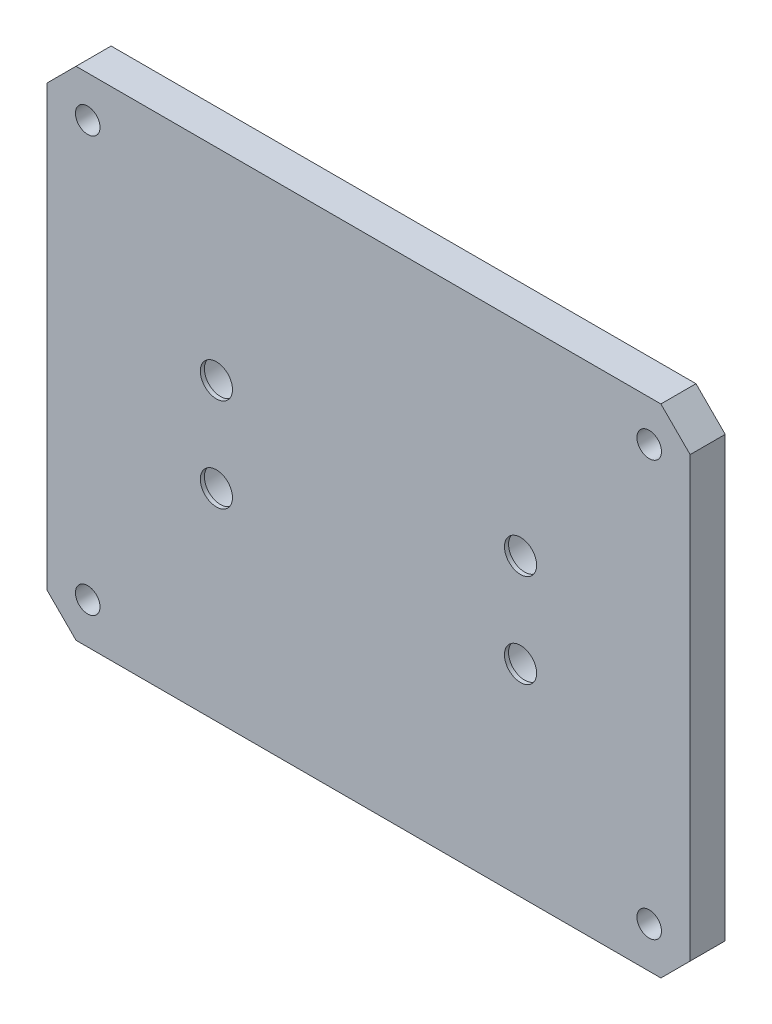
SolidWorks part; units mm, degrees
material "6061-T6 (SS)"
ref_plane "前视基准面" through (0, 0, 0) normal (0, 0, 1) x (1, 0, 0)
ref_plane "上视基准面" through (0, 0, 0) normal (0, 1, 0) x (1, 0, 0)
ref_plane "右视基准面" through (0, 0, 0) normal (1, 0, 0) x (0, 0, -1)
sketch "草图1" plane through (0, 0, 0) normal (0, 0, 1) x (1, 0, 0)
  line L1 (-76.0336, 31.3849) -> (33.9664, 31.3849)
  line L2 (-76.0336, 31.3849) -> (-76.0336, -53.6151)
  line L3 (-76.0336, -53.6151) -> (33.9664, -53.6151)
  line L4 (33.9664, 31.3849) -> (33.9664, -53.6151)
extrude "凸台-拉伸1" add sketch "草图1" along normal blind 6
chamfer "倒角1" distance 5 angle 45 4 edges at (-76.0336, 31.3849, 3) (-76.0336, -53.6151, 3) (33.9664, -53.6151, 3) (33.9664, 31.3849, 3)
hole_wizard "打孔尺寸根据内六角圆柱头螺钉的类型1" positions "草图3" profile "草图2" counterbore size "M5" standard "Gb" end condition through all
sketch "草图3" plane through (0, 0, 0) normal (0, 0, -1) x (-1, 0, 0)
  line L2 (-28.9664, 31.3849) -> (71.0336, 31.3849) construction
  line L4 (-33.9664, -48.6151) -> (-33.9664, 26.3849) construction
  point P0 (47.0336, -19.1151)
  point P3 (-4.9664, -19.1151)
  point P6 (-4.9664, -3.1151)
  point P9 (47.0336, -3.1151)
  dimension "D1" = 52
  dimension "D2" = 16
  dimension "D3" = 34.5
  dimension "D4" = 29
sketch "草图2" plane through (-47.0336, -19.1151, 0) normal (1, 0, 0) x (0, 1, 0)
  line L0 (0, 0) -> (0, 6)
  line L1 (0, 6) -> (2.75, 6)
  line L3 (2.75, 6) -> (2.75, 5.3)
  line L4 (2.75, 5.3) -> (5, 5.3)
  line L5 (5, 5.3) -> (5, 0)
  line L7 (5, 0) -> (0, 0)
  line L11 (0, -6.35) -> (0, 107.95) construction
  dimension "通孔孔直径" = 5.5
  dimension "通孔孔深度" = 6
  dimension "柱形沉头孔直径" = 10
  dimension "柱形沉头孔深度" = 5.3
hole_wizard "M5 螺纹孔1" positions "草图5" profile "草图4" tap size "M5" standard "Iso"
sketch "草图5" plane through (0, 0, 6) normal (0, 0, 1) x (1, 0, 0)
  line L0 (28.9664, 31.3849) -> (-71.0336, 31.3849) construction
  line L1 (-76.0336, 26.3849) -> (-76.0336, -48.6151) construction
  line L2 (-71.0336, -53.6151) -> (28.9664, -53.6151) construction
  line L3 (33.9664, -48.6151) -> (33.9664, 26.3849) construction
  point P0 (-69.0336, 24.3849)
  point P2 (26.9664, 24.3849)
  point P4 (26.9664, -46.6151)
  point P6 (-69.0336, -46.6151)
  dimension "D1" = 7
  dimension "D2" = 7
  dimension "D3" = 7
  dimension "D4" = 7
sketch "草图4" plane through (-69.0336, 24.3849, 6) normal (1, 0, 0) x (0, -1, 0)
  line L0 (0, 0) -> (0, 13.6618)
  line L1 (0, 13.6618) -> (2.1, 12.4)
  line L2 (2.1, 12.4) -> (2.1, 0)
  line L5 (2.1, 0) -> (0, 0)
  line L10 (0, 13.6618) -> (-2.1, 12.4) construction
  line L11 (0, -6.35) -> (0, 107.95) construction
  dimension "螺纹孔钻头直径" = 4.2
  dimension "螺纹孔钻头深度" = 12.4
  dimension "导头角度" = 118
cosmetic thread "孔螺蚊线1"
cosmetic thread "孔螺蚊线2"
cosmetic thread "孔螺蚊线3"
cosmetic thread "孔螺蚊线4"
